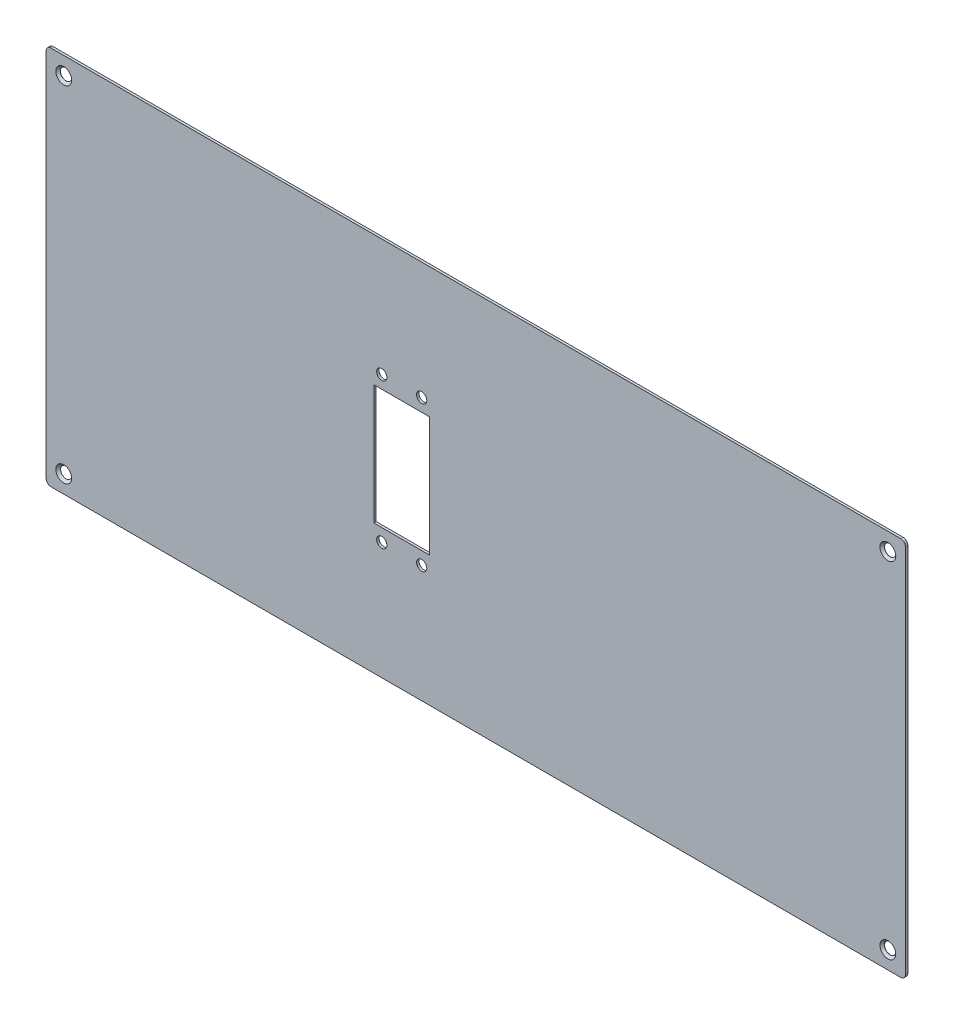
from build123d import *

# Parameters (mm, degrees)
SKETCH_1_W                       = 538.2
SKETCH_1_H                       = 238
EXTRUDE_1_DEPTH                  = 1.5
HOLE_WIZARD_7_1_7_1_1_AT_2_COUNT = 2
HOLE_WIZARD_7_1_7_1_1_AT_2_PITCH = 216
HOLE_WIZARD_7_1_7_1_1_AT_3_COUNT = 2
HOLE_WIZARD_7_1_7_1_1_AT_3_PITCH = 516.2
FILLET_1_R                       = 3
SKETCH_6_W                       = 35
SKETCH_6_H                       = 75
CUT_EXTRUDE_1_DEPTH              = 1.5
SKETCH_7_R                       = 3.2
CUT_EXTRUDE_2_DEPTH              = 1.5


with BuildPart() as part:
    # 草图1 → 凸台-拉伸1 (new body)
    with BuildSketch(Plane.XY):
        with Locations((36.480246914, 139.567901235)):
            Rectangle(SKETCH_1_W, SKETCH_1_H)
    extrude(amount=-EXTRUDE_1_DEPTH)

    # 草图2 → 孔1 (revolve, cut)
    with BuildSketch(Plane(origin=(-221.619753086, 31.567901235, 0), x_dir=(0, -1, 0), z_dir=(1, 0, 0))):
        Polygon((0, 0), (0, 1.5), (3.45, 1.5), (4.95, 0), align=None)
    revolve(axis=Axis((-221.619753086, 31.567901235, -110), (0, 0, 1)), mode=Mode.SUBTRACT)

    # 草图4 → Ø7.1 (7.1) 直径孔1 (revolve, cut)
    with BuildSketch(Plane(origin=(294.580246914, 247.567901235, 0), x_dir=(0, -1, 0), z_dir=(1, 0, 0))):
        Polygon((0, 0), (0, 1.5), (3.55, 1.5), (3.55, 1.4), (4.95, 0), align=None)
    hole_wizard_7_1_7_1_1 = revolve(axis=Axis((294.580246914, 247.567901235, 6.35), (0, 0, -1)), mode=Mode.SUBTRACT)

    # Ø7.1 (7.1) 直径孔1 at 2: Ø7.1 (7.1) 直径孔1 ×2
    with Locations(*[(0, -i * HOLE_WIZARD_7_1_7_1_1_AT_2_PITCH, 0) for i in range(1, HOLE_WIZARD_7_1_7_1_1_AT_2_COUNT)]):
        add(hole_wizard_7_1_7_1_1, mode=Mode.SUBTRACT)

    # Ø7.1 (7.1) 直径孔1 at 3: Ø7.1 (7.1) 直径孔1 ×2
    with Locations(*[(-i * HOLE_WIZARD_7_1_7_1_1_AT_3_PITCH, 0, 0) for i in range(1, HOLE_WIZARD_7_1_7_1_1_AT_3_COUNT)]):
        add(hole_wizard_7_1_7_1_1, mode=Mode.SUBTRACT)

    # 圆角1
    fillet_1_edges = [part.edges().sort_by_distance(p)[0] for p in [
        (-232.619753086, 258.567901235, -0.75),
        (305.580246914, 258.567901235, -0.75),
        (305.580246914, 20.567901235, -0.75),
        (-232.619753086, 20.567901235, -0.75),
    ]]
    fillet(fillet_1_edges, radius=FILLET_1_R)

    # 草图6 → 切除-拉伸1 (cut)
    with BuildSketch(Plane.XY):
        with Locations((-9.919753086, 139.567901235)):
            Rectangle(SKETCH_6_W, SKETCH_6_H)
    extrude(amount=-CUT_EXTRUDE_1_DEPTH, mode=Mode.SUBTRACT)

    # 草图7 → 切除-拉伸2 (cut)
    with BuildSketch(Plane.XY):
        with Locations((2.580246914, 94.067901235)):
            Circle(SKETCH_7_R)
        with Locations((-22.419753086, 94.067901235)):
            Circle(SKETCH_7_R)
        with Locations((2.580246914, 185.067901235)):
            Circle(SKETCH_7_R)
        with Locations((-22.419753086, 185.067901235)):
            Circle(SKETCH_7_R)
    extrude(amount=-CUT_EXTRUDE_2_DEPTH, mode=Mode.SUBTRACT)


solid = part.part
